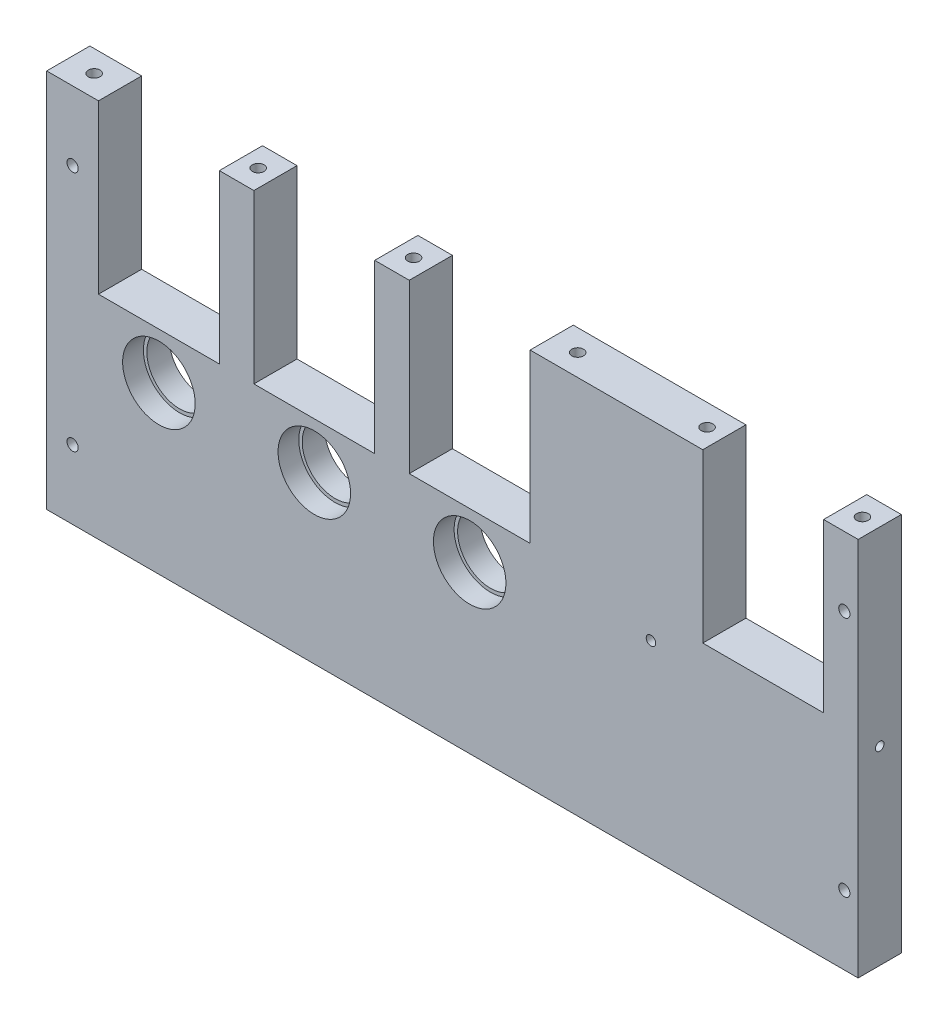
from build123d import *

# Parameters (mm, degrees)
SKETCH1_W                       = 470
SKETCH1_H                       = 260
BOSS_EXTRUDE1_DEPTH             = 12.5
SKETCH4_W                       = 70
SKETCH4_H                       = 97
CUT_EXTRUDE3_DEPTH              = 97
SKETCH5_R                       = 2.75
CUT_EXTRUDE4_DEPTH              = 97
SKETCH6_R                       = 5
CUT_EXTRUDE5_DEPTH              = 8
SKETCH7_W                       = 593.529724836
SKETCH7_H                       = 137.698896162
CUT_EXTRUDE6_DEPTH              = 40
M8_TAPPED_HOLE1_D               = 6.8
M8_TAPPED_HOLE1_DEPTH           = 20
M8_TAPPED_HOLE1_TIP             = 2.042926105
M10_TAPPED_HOLE1_D              = 8.5
M10_TAPPED_HOLE1_DEPTH          = 27.5
M10_TAPPED_HOLE1_TIP            = 2.553657631
SKETCH13_R                      = 19
CUT_EXTRUDE7_DEPTH              = 270.722079185
SKETCH14_R                      = 21
CUT_EXTRUDE8_DEPTH              = 12
LPATTERN1_COUNT                 = 3
LPATTERN1_PITCH                 = 90
SKETCH15_R                      = 3.25
CUT_EXTRUDE9_DEPTH              = 270.722079185
SKETCH16_R                      = 5.5
CUT_EXTRUDE10_DEPTH             = 10
LPATTERN2_COUNT                 = 2
LPATTERN2_PITCH                 = 447
M6_TAPPED_HOLE1_D               = 5
M6_TAPPED_HOLE1_DEPTH           = 14.5
M6_TAPPED_HOLE1_TIP             = 1.502151548
M6_TAPPED_HOLE1_ON_FACE_2_D     = 5
M6_TAPPED_HOLE1_ON_FACE_2_DEPTH = 14.5
M6_TAPPED_HOLE1_ON_FACE_2_TIP   = 1.502151548


with BuildPart() as part:
    # Sketch1 → Boss-Extrude1 (new, symmetric)
    with BuildSketch(Plane.XY):
        Rectangle(SKETCH1_W, SKETCH1_H)
    extrude(amount=BOSS_EXTRUDE1_DEPTH, both=True)

    # Sketch4 → Cut-Extrude3 (cut)
    with BuildSketch(Plane.XY.offset(12.5)):
        with Locations((-170, 81.5)):
            Rectangle(SKETCH4_W, SKETCH4_H)
        with Locations((-80, 81.5)):
            Rectangle(SKETCH4_W, SKETCH4_H)
        with Locations((10, 81.5)):
            Rectangle(SKETCH4_W, SKETCH4_H)
        with Locations((180, 81.5)):
            Rectangle(SKETCH4_W, SKETCH4_H)
    extrude(amount=-CUT_EXTRUDE3_DEPTH, mode=Mode.SUBTRACT)

    # Sketch5 → Cut-Extrude4 (cut)
    with BuildSketch(Plane.XY.offset(12.5)):
        with Locations((115, 19.25)):
            Circle(SKETCH5_R)
    extrude(amount=-CUT_EXTRUDE4_DEPTH, mode=Mode.SUBTRACT)

    # Sketch6 → Cut-Extrude5 (cut)
    with BuildSketch(Plane(origin=(0, 0, -12.5), x_dir=(-1, 0, 0), z_dir=(0, 0, -1))):
        with Locations((-115, 19.25)):
            Circle(SKETCH6_R)
    extrude(amount=-CUT_EXTRUDE5_DEPTH, mode=Mode.SUBTRACT)

    # Sketch7 → Cut-Extrude6 (cut)
    with BuildSketch(Plane(origin=(0, 0, -12.5), x_dir=(-1, 0, 0), z_dir=(0, 0, -1))):
        with Locations((25.503124985, -158.849448081)):
            Rectangle(SKETCH7_W, SKETCH7_H)
    extrude(amount=-CUT_EXTRUDE6_DEPTH, mode=Mode.SUBTRACT)

    # M8 Tapped Hole1
    with Locations(Plane(origin=(0, 130, 0), x_dir=(1, 0, 0), z_dir=(0, 1, 0))):
        with Locations((-220, 0), (225, 0), (135, 0), (-35, 0), (-125, 0), (60, 0)):
            Hole(M8_TAPPED_HOLE1_D / 2, depth=M8_TAPPED_HOLE1_DEPTH)
            with Locations((0, 0, -(M8_TAPPED_HOLE1_DEPTH + M8_TAPPED_HOLE1_TIP / 2))):  # 118° drill point
                Cone(0, M8_TAPPED_HOLE1_D / 2, M8_TAPPED_HOLE1_TIP, mode=Mode.SUBTRACT)

    # M10 Tapped Hole1
    with Locations(Plane(origin=(0, -90, 0), x_dir=(-1, 0, 0), z_dir=(0, -1, 0))):
        with Locations((-155, 0), (155, 0)):
            Hole(M10_TAPPED_HOLE1_D / 2, depth=M10_TAPPED_HOLE1_DEPTH)
            with Locations((0, 0, -(M10_TAPPED_HOLE1_DEPTH + M10_TAPPED_HOLE1_TIP / 2))):  # 118° drill point
                Cone(0, M10_TAPPED_HOLE1_D / 2, M10_TAPPED_HOLE1_TIP, mode=Mode.SUBTRACT)

    # Sketch13 → Cut-Extrude7 (cut, through all)
    with BuildSketch(Plane.XY.offset(12.5)):
        with Locations((-170, 6)):
            Circle(SKETCH13_R)
    cut_extrude7 = extrude(amount=-CUT_EXTRUDE7_DEPTH, mode=Mode.SUBTRACT)

    # Sketch14 → Cut-Extrude8 (cut)
    with BuildSketch(Plane.XY.offset(12.5)):
        with Locations((-170, 6)):
            Circle(SKETCH14_R)
    cut_extrude8 = extrude(amount=-CUT_EXTRUDE8_DEPTH, mode=Mode.SUBTRACT)

    # LPattern1: Cut-Extrude7, Cut-Extrude8 ×3
    with Locations(*[(i * LPATTERN1_PITCH, 0, 0) for i in range(1, LPATTERN1_COUNT)]):
        add(cut_extrude7, mode=Mode.SUBTRACT)
        add(cut_extrude8, mode=Mode.SUBTRACT)

    # Sketch15 → Cut-Extrude9 (cut, through all)
    with BuildSketch(Plane(origin=(0, 0, -12.5), x_dir=(-1, 0, 0), z_dir=(0, 0, -1))):
        with Locations((-227, 90)):
            Circle(SKETCH15_R)
        with Locations((-227, -50)):
            Circle(SKETCH15_R)
    cut_extrude9 = extrude(amount=-CUT_EXTRUDE9_DEPTH, mode=Mode.SUBTRACT)

    # Sketch16 → Cut-Extrude10 (cut)
    with BuildSketch(Plane(origin=(0, 0, -12.5), x_dir=(-1, 0, 0), z_dir=(0, 0, -1))):
        with Locations((-227, 90)):
            Circle(SKETCH16_R)
        with Locations((-227, -50)):
            Circle(SKETCH16_R)
    cut_extrude10 = extrude(amount=-CUT_EXTRUDE10_DEPTH, mode=Mode.SUBTRACT)

    # LPattern2: Cut-Extrude9, Cut-Extrude10 ×2
    with Locations(*[(-i * LPATTERN2_PITCH, 0, 0) for i in range(1, LPATTERN2_COUNT)]):
        add(cut_extrude9, mode=Mode.SUBTRACT)
        add(cut_extrude10, mode=Mode.SUBTRACT)

    # M6 Tapped Hole1
    with Locations(Plane(origin=(-235, 20, 0), x_dir=(0, 0, -1), z_dir=(-1, 0, 0))):
        with Locations((0, 0)):
            Hole(M6_TAPPED_HOLE1_D / 2, depth=M6_TAPPED_HOLE1_DEPTH)
            with Locations((0, 0, -(M6_TAPPED_HOLE1_DEPTH + M6_TAPPED_HOLE1_TIP / 2))):  # 118° drill point
                Cone(0, M6_TAPPED_HOLE1_D / 2, M6_TAPPED_HOLE1_TIP, mode=Mode.SUBTRACT)

    # M6 Tapped Hole1 on face 2
    with Locations(Plane(origin=(235, 20, 0), x_dir=(0, 0, 1), z_dir=(1, 0, 0))):
        with Locations((0, 0)):
            Hole(M6_TAPPED_HOLE1_ON_FACE_2_D / 2, depth=M6_TAPPED_HOLE1_ON_FACE_2_DEPTH)
            with Locations((0, 0, -(M6_TAPPED_HOLE1_ON_FACE_2_DEPTH + M6_TAPPED_HOLE1_ON_FACE_2_TIP / 2))):  # 118° drill point
                Cone(0, M6_TAPPED_HOLE1_ON_FACE_2_D / 2, M6_TAPPED_HOLE1_ON_FACE_2_TIP, mode=Mode.SUBTRACT)


solid = part.part
